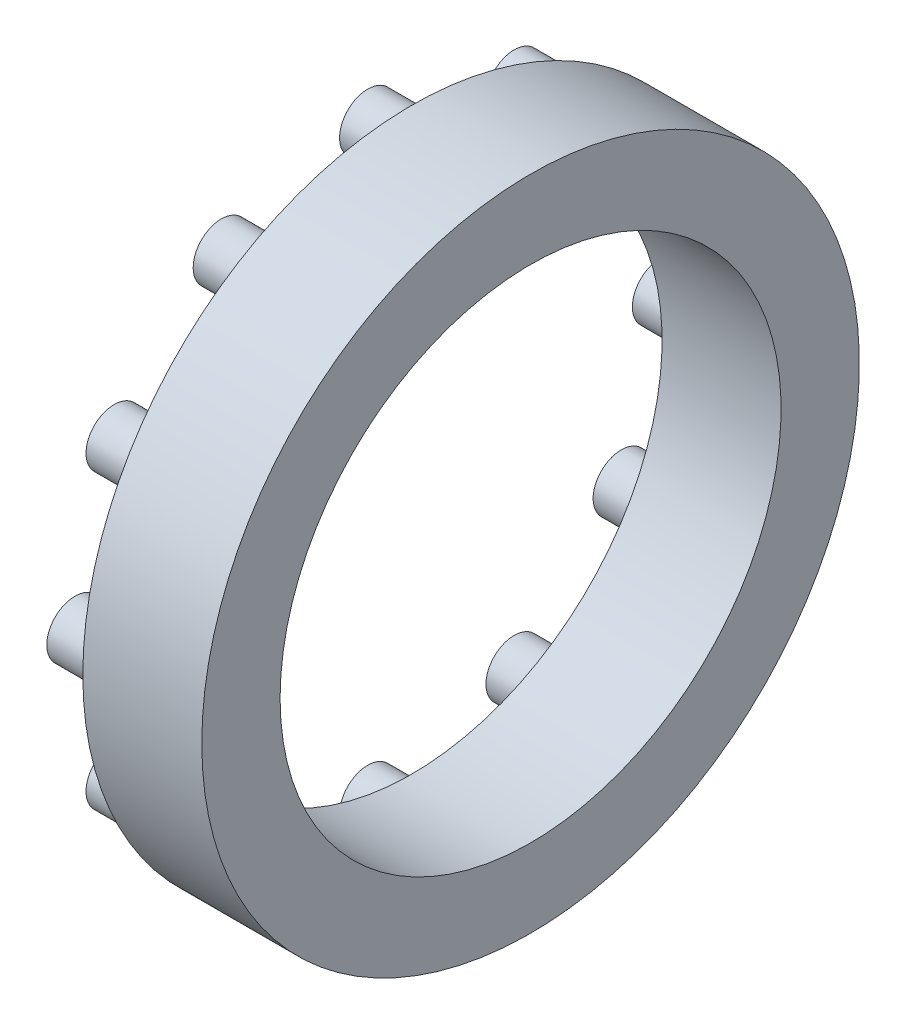
SolidWorks part; units mm, degrees
material "45"
ref_plane "Front Plane" through (0, 0, 0) normal (0, 0, 1) x (1, 0, 0)
ref_plane "Top Plane" through (0, 0, 0) normal (0, 1, 0) x (1, 0, 0)
ref_plane "Right Plane" through (0, 0, 0) normal (1, 0, 0) x (0, 0, -1)
sketch "Sketch1" plane through (0, 0, 0) normal (0, 0, 1) x (1, 0, 0)
  line L0 (0, 0) -> (110.0465, 0) construction
  line L1 (0, 0) -> (0, 105) construction
  line L2 (0, 105) -> (38, 105)
  line L3 (38, 105) -> (38, 80)
  line L4 (38, 80) -> (0, 80)
  line L5 (0, 80) -> (0, 105)
  dimension "D1" = 80
  dimension "D2" = 105
  dimension "D3" = 38
revolve "Revolve1" add sketch "Sketch1" angle 360 about L0
sketch "Sketch2" plane through (0, 0, 0) normal (-1, 0, 0) x (0, 0, 1)
  line L1 (5.715, 93.5) -> (2.8575, 98.4493)
  line L2 (2.8575, 98.4493) -> (-2.8575, 98.4493)
  line L3 (-2.8575, 98.4493) -> (-5.715, 93.5)
  line L4 (-5.715, 93.5) -> (-2.8575, 88.5507)
  line L5 (-2.8575, 88.5507) -> (2.8575, 88.5507)
  line L6 (2.8575, 88.5507) -> (5.715, 93.5)
  circle A0 centre (0, 0) radius 93.5 construction
  circle A1 centre (0, 93.5) radius 4.9493 construction
  circle A2 centre (0, 93.5) radius 9
  dimension "D1" = 187
  dimension "D3" = 18
  dimension "D2" = 11.43
extrude "Boss-Extrude1" add sketch "Sketch2" along normal blind 14
pattern_circular "CirPattern1" count 12 over 360 about axis through (0, 0, 0) along (1, 0, 0) of "Boss-Extrude1"
